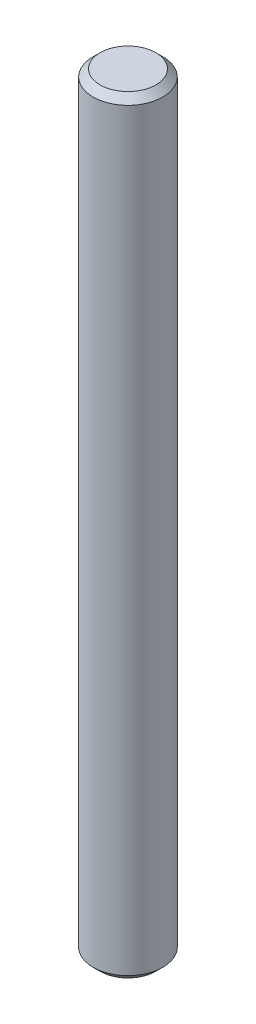
from build123d import *

# Parameters (mm, degrees)
SKETCH_1_R          = 1
EXTRUDE_1_DEPTH     = 22
CHAMFER_C0_2_1_SIZE = 0.2


with BuildPart() as part:
    # 草图1 → 凸台-拉伸1 (new body)
    with BuildSketch(Plane(origin=(0, 0, 0), x_dir=(1, 0, 0), z_dir=(0, 1, 0))):
        with Locations(Location((0, 0, 0), (0, 0, 270))):
            Circle(SKETCH_1_R)
    extrude(amount=EXTRUDE_1_DEPTH)

    # C0.2 倒角1
    chamfer_c0_2_1_edges = [part.edges().sort_by_distance(p)[0] for p in [
        (0, 0, -1),
        (0, 22, -1),
    ]]
    chamfer(chamfer_c0_2_1_edges, length=CHAMFER_C0_2_1_SIZE)


solid = part.part
